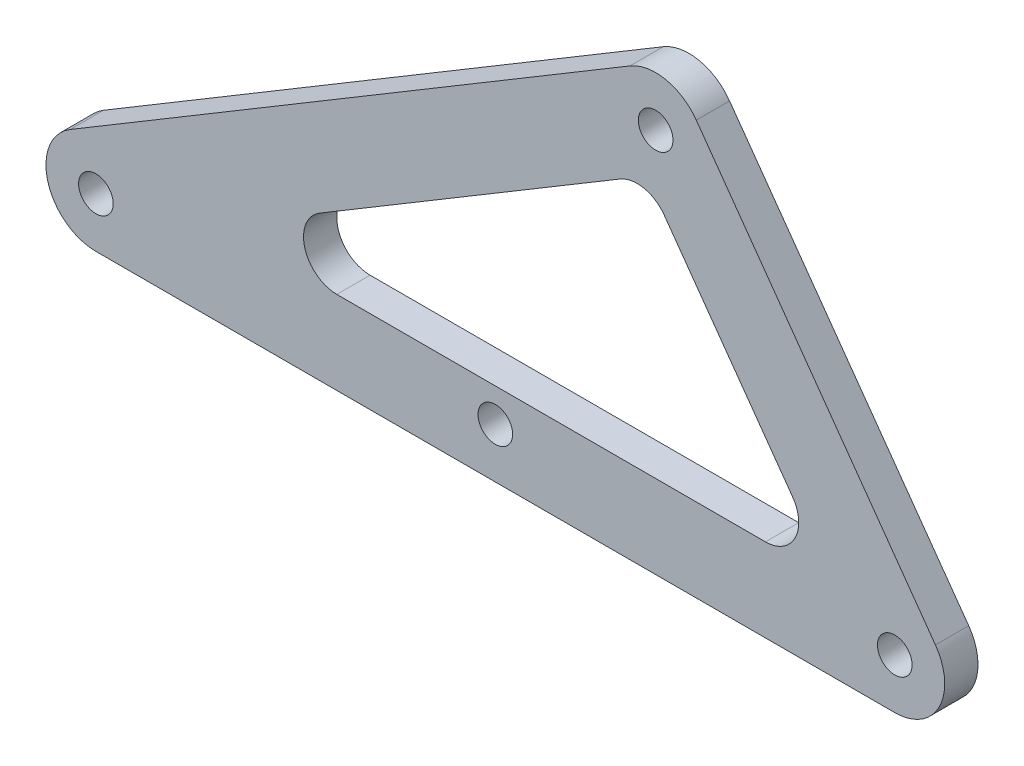
from build123d import *

# Parameters (mm, degrees)
SKETCH1_R           = 2.6
BOSS_EXTRUDE1_DEPTH = 5


with BuildPart() as part:
    # Sketch1 → Boss-Extrude1 (new body)
    with BuildSketch(Plane.XY):
        with BuildLine():
            Line((42.024169285, -45.949384393), (6.103781177, 4.358194046))
            ThreePointArc((6.103781177, 4.358194046), (1.532383005, 7.341784683), (-3.850823854, 6.435926945))
            Line((-3.850823854, 6.435926945), (-87.930468078, -43.871651494))
            ThreePointArc((-87.930468078, -43.871651494), (-91.308733105, -52.305145448), (-84.079644224, -57.807578439))
            Line((-84.079644224, -57.807578439), (-24.079629528, -57.807578439))
            Line((-24.079629528, -57.807578439), (35.920388108, -57.807578439))
            ThreePointArc((35.920388108, -57.807578439), (42.588838278, -53.740037081), (42.024169285, -45.949384393))
        make_face()
        with Locations((-84.079644224, -50.307578439)):
            Circle(SKETCH1_R, mode=Mode.SUBTRACT)
        with Locations((-24.079629528, -50.307578439)):
            Circle(SKETCH1_R, mode=Mode.SUBTRACT)
        with Locations((35.920388108, -50.307578439)):
            Circle(SKETCH1_R, mode=Mode.SUBTRACT)
        Circle(SKETCH1_R, mode=Mode.SUBTRACT)
        with BuildLine():
            Line((-5.346611856, -9.025717813), (-50.457391397, -36.016960475))
            ThreePointArc((-50.457391397, -36.016960475), (-52.709568082, -41.639289778), (-47.890175494, -45.307578439))
            Line((-47.890175494, -45.307578439), (-24.079629528, -45.307578439))
            Line((-24.079629528, -45.307578439), (16.492768241, -45.307578439))
            ThreePointArc((16.492768241, -45.307578439), (20.938401688, -42.5958842), (20.561955693, -37.402115742))
            Line((20.561955693, -37.402115742), (1.289791498, -10.41087308))
            ThreePointArc((1.289791498, -10.41087308), (-1.757807283, -8.421812655), (-5.346611856, -9.025717813))
        make_face(mode=Mode.SUBTRACT)
    extrude(amount=BOSS_EXTRUDE1_DEPTH)


solid = part.part
